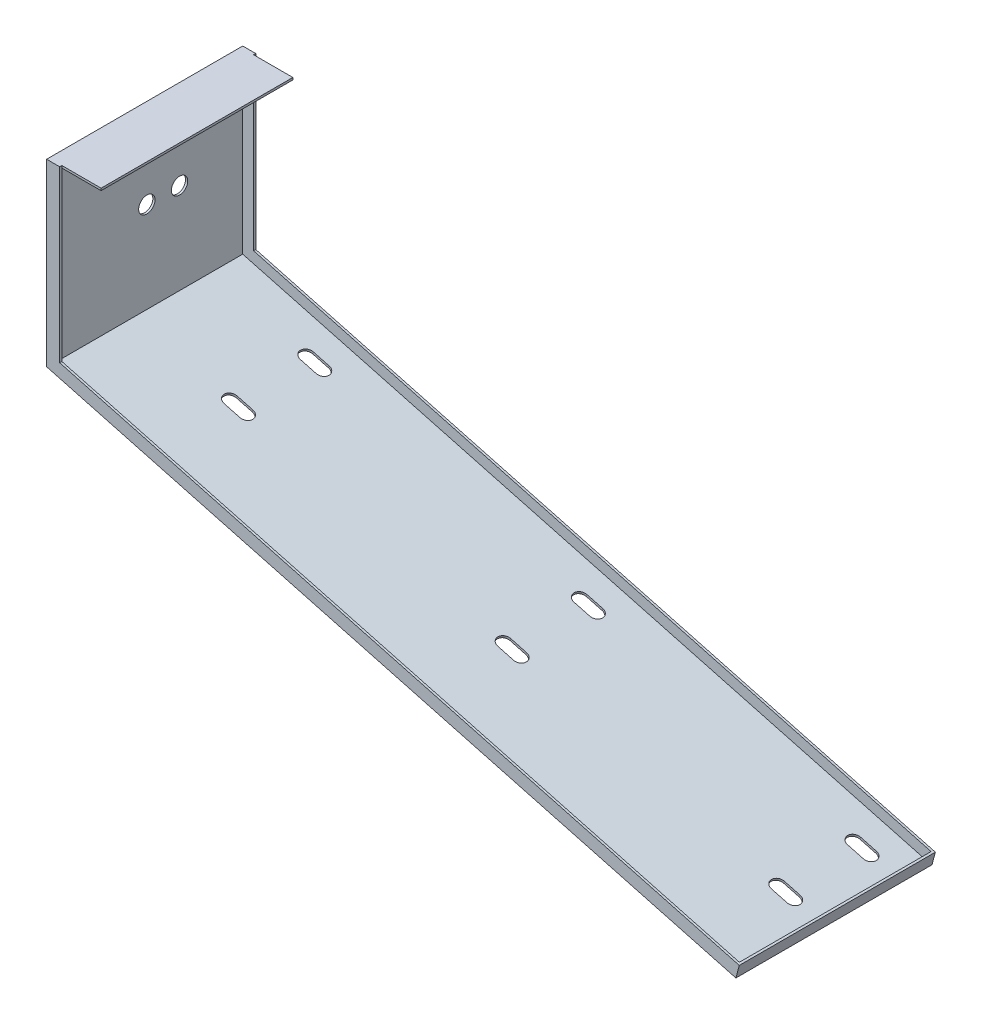
from build123d import *

# Parameters (mm, degrees)
EXTRUDE_THIN1_DEPTH  = 176
EXTRUDE_THIN2_DEPTH  = 2
EXTRUDE_THIN3_DEPTH  = 2
SKETCH4_W            = 2
SKETCH4_H            = 176
BOSS_EXTRUDE1_DEPTH  = 10
CUT_EXTRUDE1_DEPTH   = 2
LPATTERN1_COUNT      = 3
LPATTERN1_PITCH      = 260
LPATTERN1_COUNT_DIR2 = 2
LPATTERN1_PITCH_DIR2 = 70
CUT_EXTRUDE2_DEPTH   = 2
LPATTERN2_COUNT      = 2
LPATTERN2_PITCH      = 70
SKETCH7_R            = 7.5
CUT_EXTRUDE3_DEPTH   = 2
LPATTERN3_COUNT      = 2
LPATTERN3_PITCH      = 30


with BuildPart() as part:
    # Sketch1 → Extrude-Thin1 (new body)
    with BuildSketch(Plane.XY):
        Polygon((632.681416219, -169.526474542), (0, 0), (0, 165), (48, 165), (48, 163), (2, 163), (2, 1.534653976), (633.19905431, -167.59462289), align=None)
    extrude(amount=EXTRUDE_THIN1_DEPTH)

    # Sketch2 → Extrude-Thin2 (add)
    with BuildSketch(Plane.XY.offset(176)):
        Polygon((0, 165), (0, 0), (632.681416219, -169.526474542), (635.787244761, -157.935364627), (12, 9.207923856), (12, 165), align=None)
    extrude(amount=EXTRUDE_THIN2_DEPTH)

    # Sketch3 → Extrude-Thin3 (add)
    with BuildSketch(Plane(origin=(0, 0, 0), x_dir=(-1, 0, 0), z_dir=(0, 0, -1))):
        Polygon((0, 165), (0, 0), (-632.681416219, -169.526474542), (-635.787244761, -157.935364627), (-12, 9.207923856), (-12, 165), align=None)
    extrude(amount=EXTRUDE_THIN3_DEPTH)

    # Sketch4 → Boss-Extrude1 (add)
    with BuildSketch(Plane(origin=(0.51763809, 1.931851653, 0), x_dir=(0.9659258262890673, -0.25881904510252474, 0), z_dir=(0.25881904510252474, 0.9659258262890673, 0))):
        with Locations((654, -88)):
            Rectangle(SKETCH4_W, SKETCH4_H)
    extrude(amount=BOSS_EXTRUDE1_DEPTH)

    # Sketch5 → Cut-Extrude1 (cut)
    with BuildSketch(Plane(origin=(0, 0, 0), x_dir=(0.9659258262890673, -0.2588190451025247, 0), z_dir=(-0.2588190451025247, -0.9659258262890673, 0))):
        with BuildLine():
            Line((611.5, 34), (626.5, 34))
            ThreePointArc((626.5, 34), (632.5, 28), (626.5, 22))
            Line((626.5, 22), (611.5, 22))
            ThreePointArc((611.5, 22), (605.5, 28), (611.5, 34))
        make_face()
    cut_extrude1 = extrude(amount=-CUT_EXTRUDE1_DEPTH, mode=Mode.SUBTRACT)

    # LPattern1: Cut-Extrude1 3 × 2
    with Locations(*[Vector(-0.9659258262890673, 0.2588190451025247, 0) * (i * LPATTERN1_PITCH) + Vector(0, 0, 1) * (j * LPATTERN1_PITCH_DIR2) for i in range(LPATTERN1_COUNT) for j in range(LPATTERN1_COUNT_DIR2) if (i, j) != (0, 0)]):
        add(cut_extrude1, mode=Mode.SUBTRACT)

    # Sketch6 → Cut-Extrude2 (cut)
    with BuildSketch(Plane(origin=(2, 0, 0), x_dir=(0, 0, -1), z_dir=(1, 0, 0))):
        with BuildLine():
            Line((-22, 139.034653976), (-22, 124.034653976))
            ThreePointArc((-22, 124.034653976), (-28, 118.034653976), (-34, 124.034653976))
            Line((-34, 124.034653976), (-34, 139.034653976))
            ThreePointArc((-34, 139.034653976), (-28, 145.034653976), (-22, 139.034653976))
        make_face()
    cut_extrude2 = extrude(amount=-CUT_EXTRUDE2_DEPTH, mode=Mode.SUBTRACT)

    # LPattern2: Cut-Extrude2 ×2
    with Locations(*[(0, 0, i * LPATTERN2_PITCH) for i in range(1, LPATTERN2_COUNT)]):
        add(cut_extrude2, mode=Mode.SUBTRACT)

    # Sketch7 → Cut-Extrude3 (cut)
    with BuildSketch(Plane.ZY):
        with Locations((88, 85)):
            Circle(SKETCH7_R)
    cut_extrude3 = extrude(amount=-CUT_EXTRUDE3_DEPTH, mode=Mode.SUBTRACT)

    # LPattern3: Cut-Extrude3 ×2
    with Locations(*[(0, 0, -i * LPATTERN3_PITCH) for i in range(1, LPATTERN3_COUNT)]):
        add(cut_extrude3, mode=Mode.SUBTRACT)


solid = part.part
